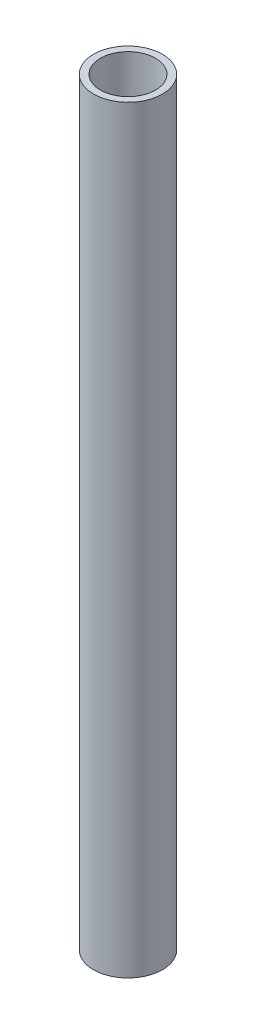
from build123d import *

# Parameters (mm, degrees)
SKETCH_2_R   = 5
SKETCH_2_R_2 = 4


with BuildPart() as part:
    # 扫描1: sweep along a path in 草图1
    with BuildLine(Plane.XY) as sweep_1_path:
        Line((0, 0), (0, 110))
    # 草图2 → 扫描1 (sweep)
    with BuildSketch(Plane(origin=(0, 0, 0), x_dir=(1, 0, 0), z_dir=(0, 1, 0))):
        Circle(SKETCH_2_R)
        Circle(SKETCH_2_R_2, mode=Mode.SUBTRACT)
    sweep(path=sweep_1_path.line)


solid = part.part
